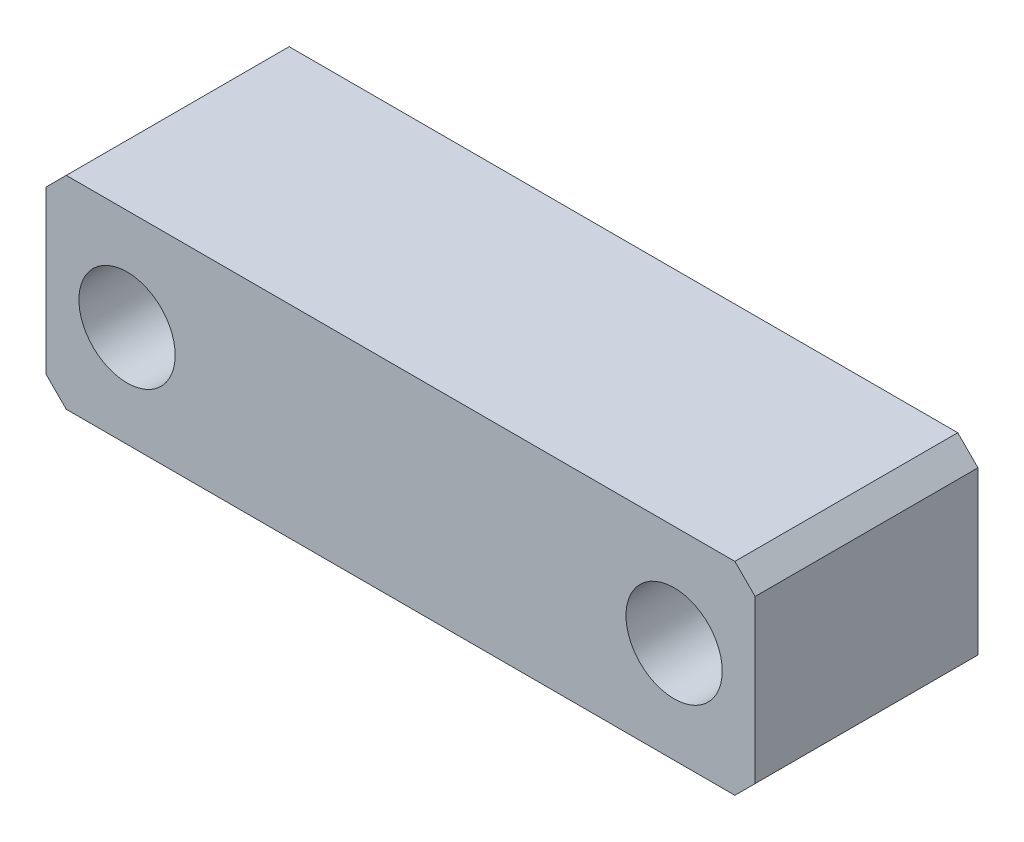
SolidWorks part; units mm, degrees
ref_plane "Front Plane" through (0, 0, 0) normal (0, 0, 1) x (1, 0, 0)
ref_plane "Top Plane" through (0, 0, 0) normal (0, 1, 0) x (1, 0, 0)
ref_plane "Right Plane" through (0, 0, 0) normal (1, 0, 0) x (0, 0, -1)
sketch "Sketch1" plane through (0, 0, 0) normal (0, 0, 1) x (1, 0, 0)
  line L0 (-24.6903, 2.0032) -> (29.3097, 2.0032) construction
  line L1 (-32.6903, 12.0032) -> (37.3097, 12.0032)
  line L2 (-32.6903, 12.0032) -> (-32.6903, -7.9968)
  line L3 (-32.6903, -7.9968) -> (37.3097, -7.9968)
  line L4 (37.3097, 12.0032) -> (37.3097, -7.9968)
  circle A0 centre (-24.6903, 2.0032) radius 2.188
  circle A1 centre (29.3097, 2.0032) radius 2.1811
  dimension "D1" = 70
  dimension "D2" = 20
  dimension "D3" = 54
  dimension "D4" = 8
extrude "Boss-Extrude1" add sketch "Sketch1" along normal blind 10 and the other way blind 12
hole_wizard "Hole1" positions "Sketch2" profile "Sketch3" legacy end condition through all
sketch "Sketch2" plane through (0, 0, 10) normal (0, 0, 1) x (1, 0, 0)
  point P2 (-24.6903, 2.0032)
  point P5 (29.3097, 2.0032)
sketch "Sketch3" plane through (-24.6903, 2.0032, 10) normal (1, 0, 0) x (0, -1, 0)
  line L0 (0, 0) -> (0, 22)
  line L1 (0, 22) -> (3, 22)
  line L2 (3, 22) -> (3, 8.5)
  line L3 (3, 8.5) -> (4.75, 8.5)
  line L4 (4.75, 8.5) -> (4.75, 0)
  line L5 (4.75, 0) -> (0, 0)
  line L6 (0, 110) -> (0, -10) construction
  dimension "直径" = 6
  dimension "深度" = 22
  dimension "柱坑直径" = 9.5
  dimension "柱坑深度" = 8.5
chamfer "Chamfer1" distance 2 angle 45 4 edges at (37.3097, -7.9968, -1) (37.3097, 12.0032, -1) (-32.6903, -7.9968, -1) (-32.6903, 12.0032, -1)
